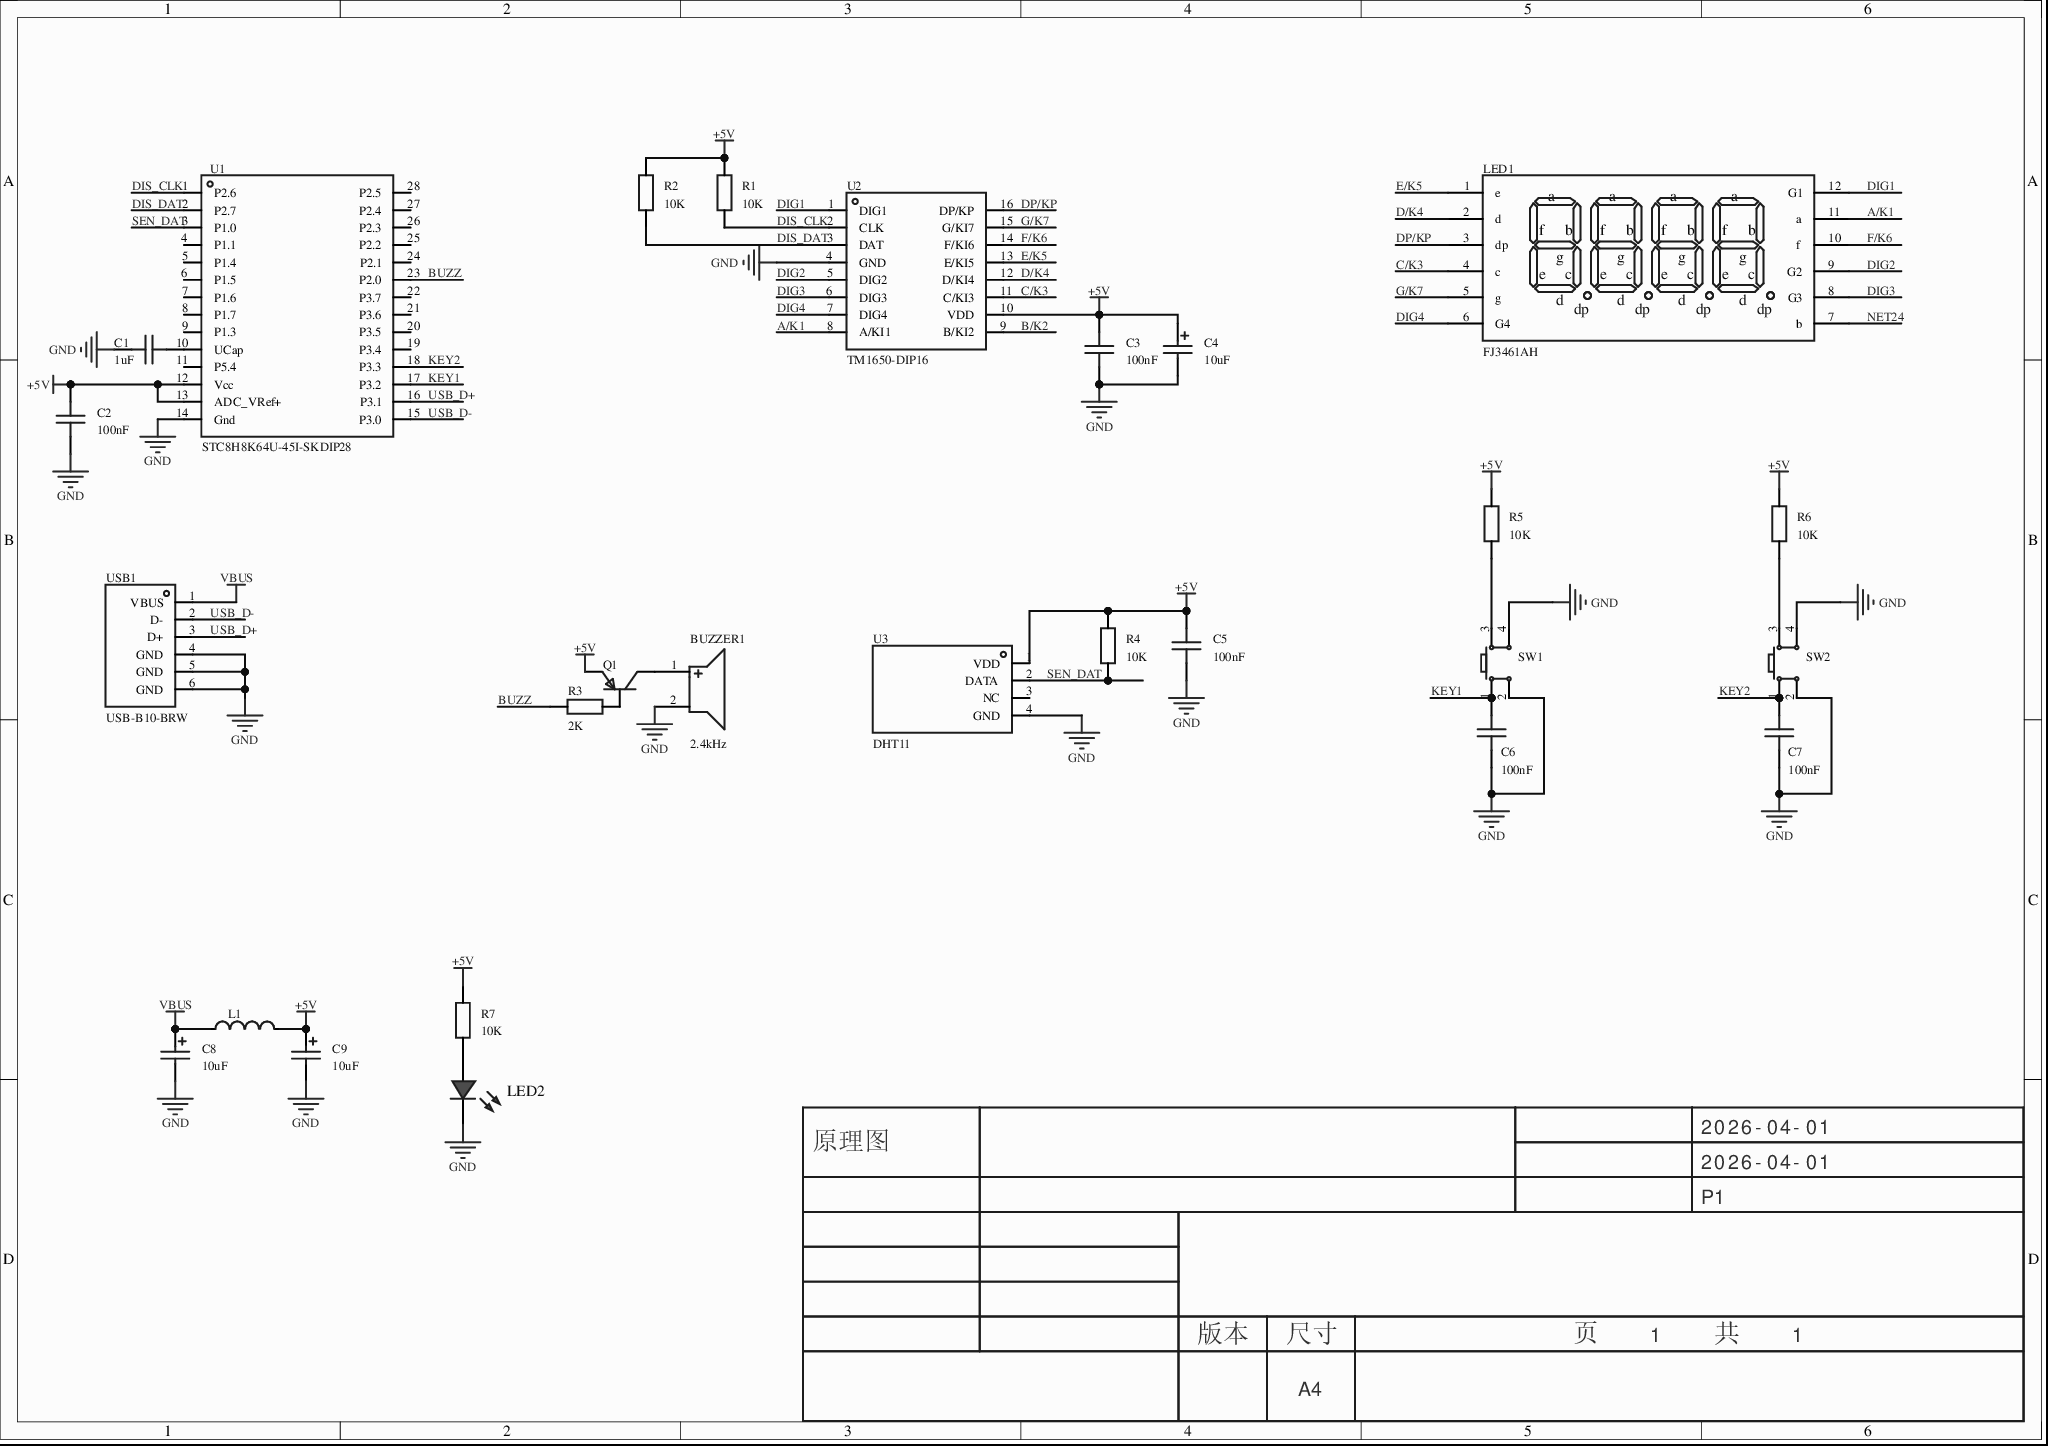
[diagram p0: MISC51906-3.schdoc]
# Altium project MISC51906-2.PrjPcb
1 sheet, 27 parts. Net scope: global (net labels, ports and power ports of the same name join across sheets).
Board file: MISC51906.pcbdoc

## Sheet MISC51906-3.schdoc
size 297 x 209 mm; Version: V1.0; @Project Name: MISC51906; @Update Date: 2026-04-01; @Create Date: 2026-04-01; @Board Name: MISC51906; @Create Time: 08:08:40; @Page Count: 1; @Page No: 1; @Schematic Name: MISC51906; @Update Time: 08:08:40; Size: A4

### Parts
BUZZER1  2.4kHz  [BUZ-TH_BD12.0-P7.60-D0.6-FD]
C1  1uF  [C0603]
C2  100nF  [C0603]
C3  100nF  [C0603]
C4  10uF  [C_Ele_SMD_3x5.4mm]
C5  100nF  [C0603]
C6  100nF  [C0603]
C7  100nF  [C0603]
C8  10uF  [C_Ele_SMD_3x5.4mm]
C9  10uF  [C_Ele_SMD_3x5.4mm]
L1  10uH  [L0603]  (value not drawn)
LED1  FJ3461AH  [LED-SEG-TH_12P-L30.0-W14.0-P2.54-S10.16-BL]
LED2  (no value)  [LED_0603]
Q1  (no value)  [S8550P_SOT]
R1  10K  [R0603]
R2  10K  [R0603]
R3  2K  [R0603]
R4  10K  [R0603]
R5  10K  [R0603]
R6  10K  [R0603]
R7  10K  [R0603]
SW1  (no value)  [SW-TH_4P-L6.0-W6.0-P4.50-LS6.5]
SW2  (no value)  [SW-TH_4P-L6.0-W6.0-P4.50-LS6.5]
U1  STC8H8K64U-45I-SKDIP28  [DIP-28_L35.3-W7.3-P2.54-LS8.4-BL]
U2  TM1650-DIP16  [DIP-16_L19.3-W6.4-P2.54-LS8.0-BL]
U3  DHT11  [SENSOR-TH_DHT11]
USB1  USB-B10-BRW  [USB-B-TH_USB-B10-BRW]

### Nets
+5V: C2.2 C3.2 C4.1 C5.2 C9.1 L1.2 Q1.2(E) R1.2 R2.2 R4.2 R5.2 R6.2 R7.2 U1.12(Vcc) U1.13(ADC_VRef+) U2.10(VDD) U3.1(VDD)
GND: BUZZER1.2 C1.1 C2.1 C3.1 C4.2 C5.1 C6.1 C7.1 C8.2 C9.2 LED2.1(C) SW1.2 SW1.4 SW2.2 SW2.4 U1.14(Gnd) U2.4(GND) U3.4(GND) USB1.4(GND) USB1.5(GND) USB1.6(GND)
VBUS: C8.1 L1.1 USB1.1(VBUS)
A/K1: LED1.11(a) U2.8(A/KI1)
B/K2: U2.9(B/KI2)
BUZZ: R3.1 U1.23(P2.0)
C/K3: LED1.4(c) U2.11(C/KI3)
D/K4: LED1.2(d) U2.12(D/KI4)
DIG1: LED1.12(G1) U2.1(DIG1)
DIG2: LED1.9(G2) U2.5(DIG2)
DIG3: LED1.8(G3) U2.6(DIG3)
DIG4: LED1.6(G4) U2.7(DIG4)
DIS_CLK: R1.1 U1.1(P2.6) U2.2(CLK)
DIS_DAT: R2.1 U1.2(P2.7) U2.3(DAT)
DP/KP: LED1.3(dp) U2.16(DP/KP)
E/K5: LED1.1(e) U2.13(E/KI5)
F/K6: LED1.10(f) U2.14(F/KI6)
G/K7: LED1.5(g) U2.15(G/KI7)
KEY1: C6.2 SW1.1 U1.17(P3.2)
KEY2: C7.2 SW2.1 U1.18(P3.3)
NET24: LED1.7(b)
SEN_DAT: R4.1 U1.3(P1.0) U3.2(DATA)
USB_D+: U1.16(P3.1) USB1.3(D+)
USB_D-: U1.15(P3.0) USB1.2(D-)
NetBUZZER1_1: BUZZER1.1 Q1.3(C)
NetC1_2: C1.2 U1.10(UCap)
NetLED2_2: LED2.2(A) R7.1
NetQ1_1: Q1.1(B) R3.2
NetR5_1: R5.1 SW1.3
NetR6_1: R6.1 SW2.3

Not connected (* = marked no-connect by the designer): U1 4(P1.1)* 5(P1.4)* 6(P1.5)* 7(P1.6)* 8(P1.7)* 9(P1.3)* 11(P5.4)* 19(P3.4)* 20(P3.5)* 21(P3.6)* 22(P3.7)* 24(P2.1)* 25(P2.2)* 26(P2.3)* 27(P2.4)* 28(P2.5)*; U3 3(NC)*

### Layout directives
differential pair; Symbol: Differential-Pairs-Flag; Device: Differential-Pairs-Flag: USB_D+, USB_D-

### Notes on the sheet
- 2026-04-01
- 原理图
- P1
- 版本
- 尺寸
- A4
- 页    1    共    1

### Library data of the parts
BUZZER1 = TMB12A05: 驱动方式:有源(内含驱动线路);构造类型:电磁式;频率:2.4kHz;声压(SPL):88dB;; Manufacturer: YUEXIN(悦馨); Symbol: TMB12A05_C781860; AddInBom: yes; ModelId: 16ab50e14c5b4f2c986c135bdba60e370819f05c4eef4c71ace90d822a990e87; ModelName: BUZ-TH_D12.0-H9.5-P7.60; ModelTransform: 472.44,472.176,0,90,0,0,-0.787,0,-177.165; Voltage - Supply: 4V~8V; Current Consumption: 30mA; Sound Pressure Level(SPL): 88dB; Device: TMB12A05; LCSC Part Name: 有源电磁式蜂鸣器; SupplierPart: C781860; ManufacturerPart: TMB12A05; Supplier Footprint: 插件,D=12mm; JLCPCB Part Class: Extended Part; Datasheet: https://item.szlcsc.com/datasheet/TMB12A05/834376.html; Supplier: LCSC; ConvertToPcb: yes; FootprintName: BUZ-TH_BD12.0-P7.60-D0.6-FD; Driver Circuitry: 有源(内含驱动线路); Technology: 电磁式; Value: 2.4kHz; Diameter(φD): 12mm; Length: -; Width: -; Height: 9.5mm; Operating Temperature: -30℃~+85℃
C1-C3 C5-C7 = CAP_0603: Symbol: Capacitance; ConvertToPcb: yes; ModelId: ac125912035d415993ca9572d50418b10819f05c4eef4c71ace90d822a990e87; ModelName: C0603_L1.6-W0.8-H0.8; ModelTransform: 62.992,31.496,0,0,0,0,0,0,0; Device: CAP_0603; AddInBom: yes; Supplier Footprint: 0603; FootprintName: C0603
  C1: Value: 1uF
  C2 C3 C5-C7: Value: 100nF
C4 C8 C9 = C_Ele_SMD_3x5.4mm: Symbol: CAP; AddInBom: yes; ModelId: 0132c3d3fdbf4fd987f710a97e7a5b5d0819f05c4eef4c71ace90d822a990e87; ModelName: CAP-SMD_BD3.0-L3.3-W3.3-H5.3; ModelTransform: 129.9,149.58,209.06,-90,0,0,0,0,0; Device: C_Ele_SMD_3x5.4mm; Supplier Footprint: SMD,3x5.4mm; ConvertToPcb: yes; FootprintName: C_Ele_SMD_3x5.4mm; Value: 10uF
L1 = L_0603: Symbol: SDFL1608S100KTF; AddInBom: yes; ModelId: 2bc5ec593d464d6ba9807aec0b5673c20819f05c4eef4c71ace90d822a990e87; ModelName: L0603_L1.6-W0.8-H0.5_BEAD; ModelTransform: 62.992,31.496,0,180,0,0,0.094,0.629,0; Device: L_0603; Supplier Footprint: L0603; ConvertToPcb: yes; FootprintName: L0603; Value: 10uH
LED1 = FJ3461AH: 数码管位数:4位;字符尺寸(英寸):0.36;耗散功率(Pd):-;发光颜色:红色;LED极性:共阴极;; Manufacturer: 志浩; AddInBom: yes; ModelId: 413f3531b06c40ffa975bee3b430fbb40819f05c4eef4c71ace90d822a990e87; ModelName: LED-SEG-TH_0.36-4P; ModelTransform: 1181.1,551.18,0,0,0,0,-0.001,-0.001,-137.795; Number of Characters: 4位; Digit/Alpha Size(inch): 0.36; Illumination Color: 红色; LED Polarity: 共阴极; Symbol: FJ3461AH; Device: FJ3461AH; LCSC Part Name: 4位0.36英寸红色数码管 共阴极; SupplierPart: C10708; ManufacturerPart: FJ3461AH; Supplier Footprint: 插件; JLCPCB Part Class: Extended Part; Datasheet: https://item.szlcsc.com/datasheet/FJ3461AH/11252.html; Supplier: LCSC; ConvertToPcb: yes; FootprintName: LED-SEG-TH_12P-L30.0-W14.0-P2.54-S10.16-BL; Display Type: -; Pd - Power Dissipation: -
LED2 = LED_0603-R: Symbol: LED_R; Convert to PCB: yes; 3D Model: dd8257b0d61a4cd7b68939a056e080950819f05c4eef4c71ace90d822a990e87; 3D Model Transform: 58.72,29.4,22.03,0,0,0,0,0,0; ModelName: LED-0603_R; Device: LED_0603-R; Add into BOM: yes; Supplier Footprint: 0603; FootprintName: LED_0603
Q1 = S8550_SOT_PNP: Symbol: PNP; ConvertToPcb: yes; ModelId: 9c0df02d6f3e44e889da37f3e5bf54960819f05c4eef4c71ace90d822a990e87; ModelName: SOT-23-3_L2.9-W1.4-P1.90-LS2.5-BR; ModelTransform: 98.43,114.17,37.91,0,0,0,0,0,0; Device: S8550_SOT_PNP; AddInBom: yes; Supplier Footprint: SOT-23; FootprintName: S8550P_SOT
R1-R7 = Res_0603: Symbol: 电阻; ConvertToPcb: yes; ModelId: fc143cca1e79419f9cd78b61e9279f080819f05c4eef4c71ace90d822a990e87; ModelTransform: 31.8897,63.7794,0,90,0,0,0,0,0; Device: Res_0603; AddInBom: yes; Supplier Footprint: 0603; FootprintName: R0603; ModelName: R0603
  R1 R2 R4-R7: Value: 10K
  R3: Value: 2K
SW1 SW2 = Key_TH_6x6x6: 触点电流:50mA;额定电压(DC):12V;绝缘电阻:100MΩ;电路结构:单刀单掷;安装方式:直插;按钮形状:圆形按钮;按钮/盖帽颜色:黑色;作用力:260gf@±30gf;工作温度:-25℃~+70℃;引脚样式:PC引脚;开关长度:6mm;开关宽度:6mm;开关高度:6mm;带支架:否;; Symbol: 轻触按键; AddInBom: yes; ModelId: 20eee248bc684ccd8cbdbb1d0d91ec6f0819f05c4eef4c71ace90d822a990e87; ModelName: SW-TH_4P-L6.0-W6.0-H5.0-LS6.5-P4.50; ModelTransform: 236.22,323.03,0,90,0,0,0,0,-137.795; Device: Key_TH_6x6x6; ConvertToPcb: yes; FootprintName: SW-TH_4P-L6.0-W6.0-P4.50-LS6.5; Supplier Footprint: 插件
U1 = STC8H8K64U-45I-SKDIP28: Manufacturer: STC; AddInBom: yes; ModelId: 5a9815e6937c481f9b5a663ef692cbff0819f05c4eef4c71ace90d822a990e87; ModelTransform: 1389.76116,338.582,0,0,0,0,0,0,-118.11; Symbol: STC8H8K64U-45I-SKDIP28; Device: STC8H8K64U-45I-SKDIP28; LCSC Part Name: 宽电压/高速/高可靠/低功耗/强抗静电/较强抗干扰的新一代 8051 单片机; SupplierPart: C7543848; ManufacturerPart: STC8H8K64U-45I-SKDIP28; Supplier Footprint: SKDIP28; JLCPCB Part Class: Extended Part; Datasheet: https://atta.szlcsc.com/upload/public/pdf/source/20250313/1FF371FFB32C4E4D51E663CECCBEC974.pdf; Supplier: LCSC; ConvertToPcb: yes; FootprintName: DIP-28_L35.3-W7.3-P2.54-LS8.4-BL; ModelName: DIP-28_L35.3-W7.3-P2.54-LS8.4-BL
U2 = TM1650-DIP16: 类型:-;工作电压(DC):3V~5.5V;开关频率:-;通道数:-;输出电压:-;输出电流:150mA;调光:-;拓扑结构:-;; Manufacturer: TM(天微); AddInBom: yes; ModelId: 0b97c16a330048e59699e00b4c3cf2920819f05c4eef4c71ace90d822a990e87; ModelTransform: 759.841,322.44,0,0,0,0,0,0,-125.984; Output Current: 150mA; Symbol: TM1650-DIP16; Device: TM1650-DIP16; LCSC Part Name: LED（发光二极管显示器）; SupplierPart: C22767315; ManufacturerPart: TM1650-DIP16; Supplier Footprint: DIP-16; JLCPCB Part Class: Extended Part; Datasheet: https://item.szlcsc.com/datasheet/TM1650-DIP16/24494228.html; Supplier: LCSC; ConvertToPcb: yes; FootprintName: DIP-16_L19.3-W6.4-P2.54-LS8.0-BL; ModelName: DIP-16_L19.3-W6.4-P2.54-LS8.0-BL; Type: -; Voltage - Input(DC): 3V~5.5V; Frequency - Switching: -; Number of Channels: -; Output Voltage: -; Dimming: -; Features: -; Voltage - Input(AC): -; Topology: -; Operating temperature: -40℃~+85℃; Switch Tube (Built-In/External): -; Constant Current Accuracy: -
U3 = DHT11: 温度范围:-20℃~+60℃;湿度范围:5%RH~95%RH;湿度精度:±5%RH;; Manufacturer: 广州奥松; AddInBom: yes; ModelId: 6dde47d4d8bf4fa598dffcc067449c1d0819f05c4eef4c71ace90d822a990e87; ModelTransform: 236.25937,492.125,0,270,0,0,0,-11.811,-196.85; Voltage - Supply: 3.3V~5.5V; Current - Supply: 1mA; Humidity Tolerance: ±5%RH; Temperature Tolerance: ±2℃; Symbol: DHT11; Device: DHT11; LCSC Part Name: 新款电容式数字温湿度传感器,老款已停产16.1x12.6x5.8mm DHT11  电容式传感器; SupplierPart: C117051; ManufacturerPart: DHT11; Supplier Footprint: SIP-4; JLCPCB Part Class: Extended Part; Datasheet: https://item.szlcsc.com/datasheet/DHT11/118309.html; Supplier: LCSC; ConvertToPcb: yes; FootprintName: SENSOR-TH_DHT11; ModelName: SENSOR-TH_DHT11; Temperature Range: -20℃~+60℃; Humidity: 5%RH~95%RH
USB1 = USB-B10-BRW: 连接器类型:Type-B;协议标准:USB 2.0;公母:母;安装方式:弯插;触点数量:4P;端口数量:1;额定电流 - 电源:1.5A;工作温度:-20℃~+70℃;; Manufacturer: XUNPU(讯普); AddInBom: yes; ModelId: 44436f1d19854c47bde1092be1a59de30819f05c4eef4c71ace90d822a990e87; ModelTransform: 562.447,643.7,0,0,0,0,-0.002,-181.892,-125.984; Connector Type: Type-B; Protocol Standard: USB 2.0; Gender: 母; Number of Contacts: 4P; Number of Ports: 1; Current Rating-Power: 1.5A; Voltage Rating: 30V; Detection color: 白色; Symbol: USB-B10-BRW; Device: USB-B10-BRW; LCSC Part Name: Type-B 母 弯插; SupplierPart: C720549; ManufacturerPart: USB-B10-BRW; Supplier Footprint: 弯插; JLCPCB Part Class: Extended Part; Datasheet: https://item.szlcsc.com/datasheet/USB-B10-BRW/763556.html; Supplier: LCSC; ConvertToPcb: yes; FootprintName: USB-B-TH_USB-B10-BRW; ModelName: USB-B-TH_USB-B10-BRW; Mounting Type: 弯插; Length: 16.3mm; Operating Temperature: -20℃~+70℃